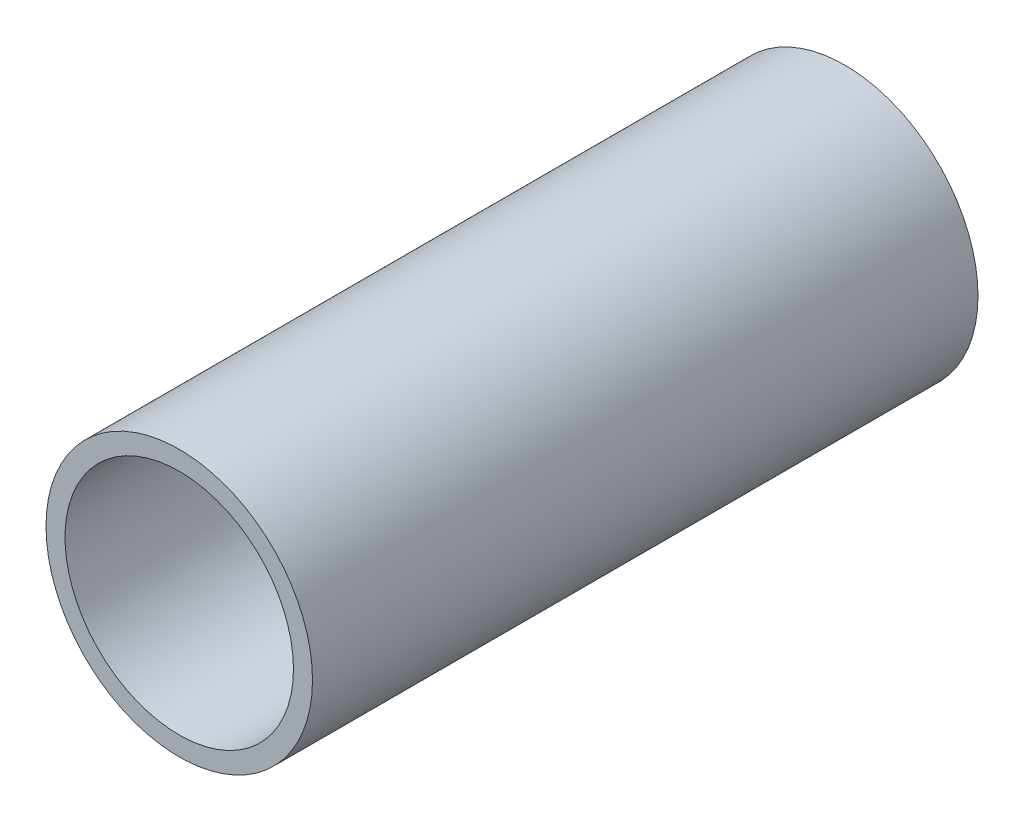
SolidWorks part; units mm, degrees
ref_plane "前视基准面" through (0, 0, 0) normal (0, 0, 1) x (1, 0, 0)
ref_plane "上视基准面" through (0, 0, 0) normal (0, 1, 0) x (1, 0, 0)
ref_plane "右视基准面" through (0, 0, 0) normal (1, 0, 0) x (0, 0, -1)
sketch "草图1" plane through (0, 0, 0) normal (0, 0, 1) x (1, 0, 0)
  circle A0 centre (0, 0) radius 38.1
  circle A1 centre (0, 0) radius 44.45
  dimension "D1" = 88.9
  dimension "D2" = 76.2
extrude "凸台-拉伸1" add sketch "草图1" along normal mid plane 222
